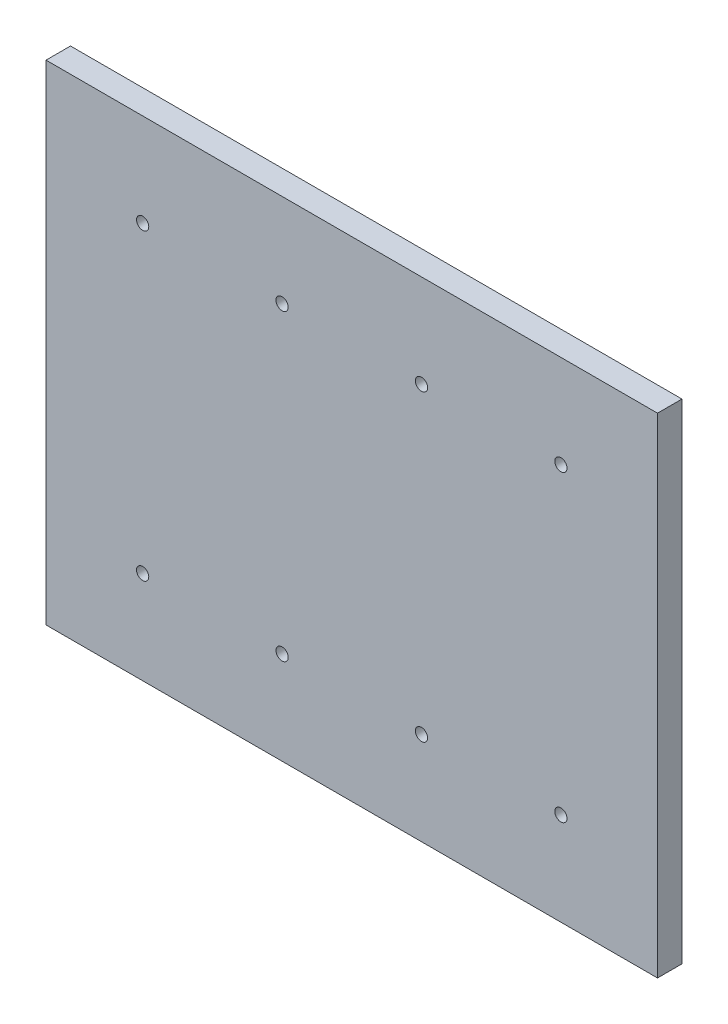
from build123d import *

# Parameters (mm, degrees)
SKETCH1_W           = 250
SKETCH1_H           = 200
BOSS_EXTRUDE1_DEPTH = 10
M6_TAPPED_HOLE1_D   = 5


with BuildPart() as part:
    # Sketch1 → Boss-Extrude1 (new body)
    with BuildSketch(Plane.XY):
        Rectangle(SKETCH1_W, SKETCH1_H)
    extrude(amount=BOSS_EXTRUDE1_DEPTH)

    # M6 Tapped Hole1 (through all)
    with Locations(Plane.XY.offset(10)):
        with Locations((-85.5, 62), (-28.5, 62), (85.5, 62), (28.5, 62), (28.5, -62), (85.5, -62), (-28.5, -62), (-85.5, -62)):
            Hole(M6_TAPPED_HOLE1_D / 2)


solid = part.part
